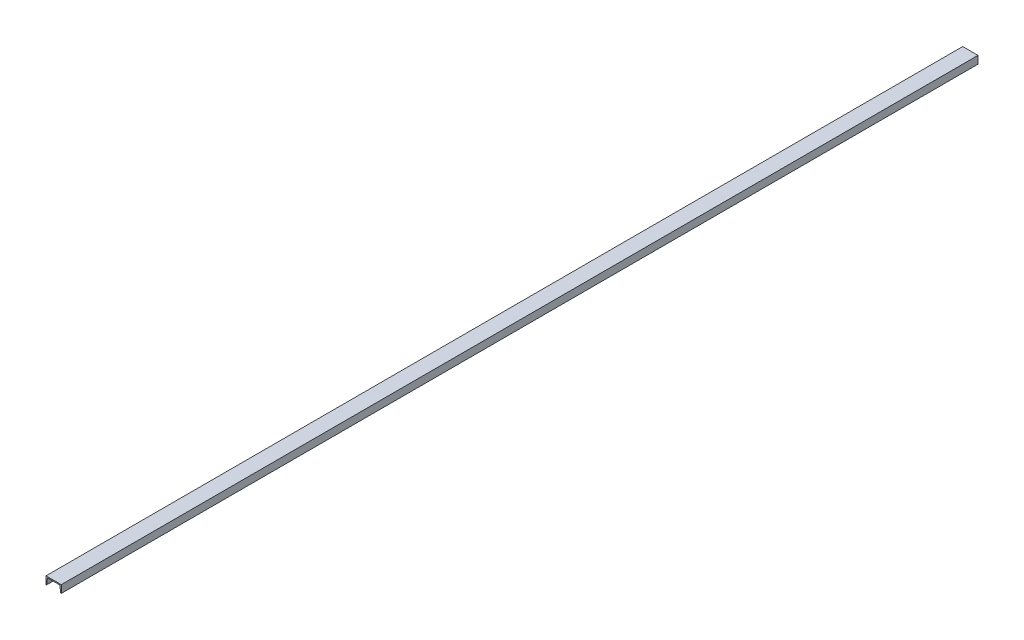
SolidWorks part; units mm, degrees
material "普通碳钢"
ref_plane "Front Plane" through (0, 0, 0) normal (0, 0, 1) x (1, 0, 0)
ref_plane "Top Plane" through (0, 0, 0) normal (0, 1, 0) x (1, 0, 0)
ref_plane "Right Plane" through (0, 0, 0) normal (1, 0, 0) x (0, 0, -1)
sketch "Sketch1" plane through (0, 0, 0) normal (0, 0, 1) x (1, 0, 0)
  line L0 (0, 0) -> (0, 50)
  line L1 (0, 50) -> (100, 50)
  line L2 (100, 50) -> (100, 0)
  line L3 (0, 0) -> (2.5485, 0)
  line L4 (4.5356, 1.7732) -> (8.7527, 38.7239)
  line L5 (13.7205, 43.1569) -> (86.2795, 43.1569)
  line L6 (50, 50) -> (50, 36.5447) construction
  line L7 (100, 0) -> (97.4515, 0)
  line L8 (95.4644, 1.7732) -> (91.2473, 38.7239)
  arc A0 (8.7527, 38.7239) -> (13.7205, 43.1569) centre (13.7205, 38.1569) cw
  arc A1 (4.5356, 1.7732) -> (2.5485, 0) centre (2.5485, 2) cw
  arc A2 (91.2473, 38.7239) -> (86.2795, 43.1569) centre (86.2795, 38.1569) ccw
  arc A3 (95.4644, 1.7732) -> (97.4515, 0) centre (97.4515, 2) ccw
  point P15 (50, 43.1569)
  dimension "D4" = 5
  dimension "D5" = 2
  dimension "D1" = 100
  dimension "D3" = 50
extrude "Boss-Extrude1" add sketch "Sketch1" along normal blind 6000
